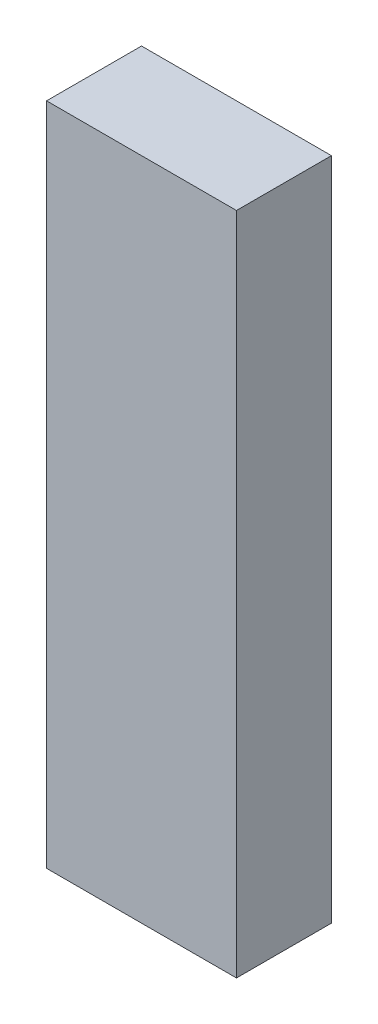
from build123d import *

# Parameters (mm, degrees)
SKETCH_1_W      = 20
SKETCH_1_H      = 70
EXTRUDE_1_DEPTH = 10


with BuildPart() as part:
    # 草图1 → 凸台-拉伸1 (new body)
    with BuildSketch(Plane.XY):
        with Locations((10, 35)):
            Rectangle(SKETCH_1_W, SKETCH_1_H)
    extrude(amount=EXTRUDE_1_DEPTH)


solid = part.part
